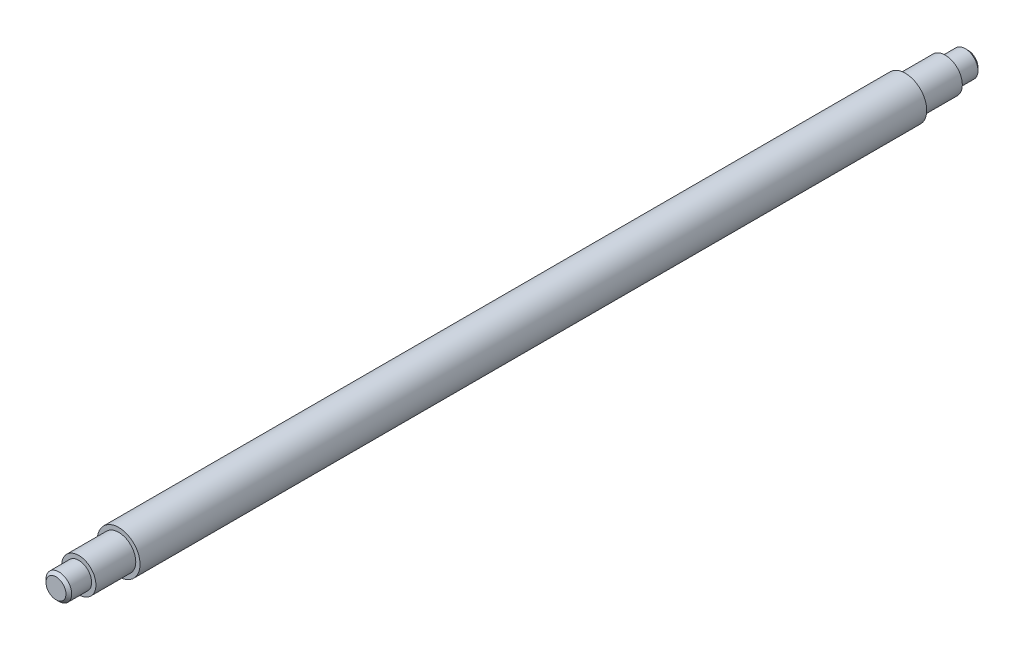
SolidWorks part; units mm, degrees
ref_plane "前视基准面" through (0, 0, 0) normal (0, 0, 1) x (1, 0, 0)
ref_plane "上视基准面" through (0, 0, 0) normal (0, 1, 0) x (1, 0, 0)
ref_plane "右视基准面" through (0, 0, 0) normal (1, 0, 0) x (0, 0, -1)
sketch "草图1" plane through (0, 0, 0) normal (0, 0, 1) x (1, 0, 0)
  circle A0 centre (0, 0) radius 4.5
  dimension "D1" = 9
extrude "凸台-拉伸1" add sketch "草图1" along normal blind 8
sketch "草图2" plane through (0, 0, 8) normal (0, 0, 1) x (1, 0, 0)
  circle A0 centre (0, 0) radius 6
extrude "凸台-拉伸2" add sketch "草图2" along normal blind 14
sketch "草图3" plane through (0, 0, 22) normal (0, 0, 1) x (1, 0, 0)
  circle A0 centre (0, 0) radius 7.5
extrude "凸台-拉伸3" add sketch "草图3" along normal blind 276
sketch "草图4" plane through (0, 0, 298) normal (0, 0, 1) x (1, 0, 0)
  circle A0 centre (0, 0) radius 6
extrude "凸台-拉伸4" add sketch "草图4" along normal blind 14
sketch "草图5" plane through (0, 0, 312) normal (0, 0, 1) x (1, 0, 0)
  circle A0 centre (0, 0) radius 4.5
extrude "凸台-拉伸5" add sketch "草图5" along normal blind 8
chamfer "倒角1" distance 1 angle 45 2 edges at (4.5, 0, 0) (4.5, 0, 320)
ref_plane "基准面1" through (0, 0, 273) normal (0, 0, 1) x (1, 0, 0)
sketch "草图7" plane through (0, 0, 273) normal (0, 0, 1) x (1, 0, 0)
  circle A0 centre (0, 0) radius 8
extrude "凸台-拉伸7" [suppressed] add sketch "草图7" against normal blind 145
ref_plane "基准面2" through (0, 0, 160) normal (0, 0, 1) x (1, 0, 0)
mirror "镜向1" [suppressed] about plane through (0, 0, 160) normal (0, 0, 1)
